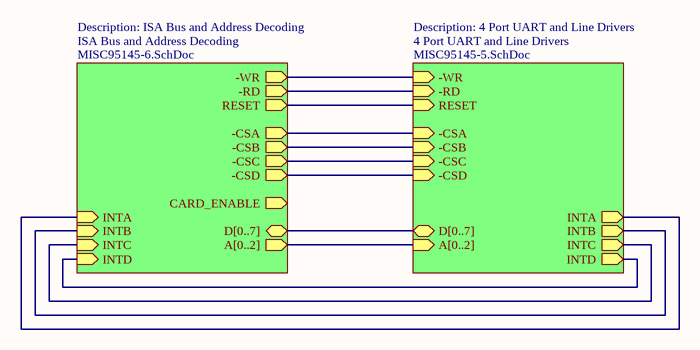
[diagram p0: MISC95145.SchDoc]
# Altium project MISC95145.PRJPCB
3 sheets, 36 parts. Net scope: hierarchical (ports join the sheet entries above them; power ports are global).
Board file: MISC95145.PcbDoc
Sheets:
  MISC95145.SchDoc
    4 Port UART and Line Drivers = MISC95145-5.SchDoc
    ISA Bus and Address Decoding = MISC95145-6.SchDoc

## Sheet MISC95145.SchDoc
size A

### Sub-sheets
4 Port UART and Line Drivers = MISC95145-5.SchDoc: A[0..2] (in), D[0..7] (bidir), -CSA (in), -CSB (in), -CSC (in), -CSD (in), INTA (out), INTB (out), INTC (out), INTD (out), -RD (in), -WR (in), RESET (in)  | Description: 4 Port UART and Line Drivers
ISA Bus and Address Decoding = MISC95145-6.SchDoc: D[0..7] (bidir), -WR (out), -RD (out), RESET (out), A[0..2] (out), -CSA (out), -CSB (out), -CSC (out), -CSD (out), CARD_ENABLE (out), INTB (in), INTC (in), INTD (in), INTA (in)  | Description: ISA Bus and Address Decoding

### Nets
-CSA: sheet 4 Port UART and Line Drivers/-CSA, sheet ISA Bus and Address Decoding/-CSA
-CSB: sheet 4 Port UART and Line Drivers/-CSB, sheet ISA Bus and Address Decoding/-CSB
-CSC: sheet 4 Port UART and Line Drivers/-CSC, sheet ISA Bus and Address Decoding/-CSC
-CSD: sheet 4 Port UART and Line Drivers/-CSD, sheet ISA Bus and Address Decoding/-CSD
-RD: sheet 4 Port UART and Line Drivers/-RD, sheet ISA Bus and Address Decoding/-RD
-WR: sheet 4 Port UART and Line Drivers/-WR, sheet ISA Bus and Address Decoding/-WR
INTA: sheet 4 Port UART and Line Drivers/INTA, sheet ISA Bus and Address Decoding/INTA
INTB: sheet 4 Port UART and Line Drivers/INTB, sheet ISA Bus and Address Decoding/INTB
INTC: sheet 4 Port UART and Line Drivers/INTC, sheet ISA Bus and Address Decoding/INTC
INTD: sheet 4 Port UART and Line Drivers/INTD, sheet ISA Bus and Address Decoding/INTD
RESET: sheet 4 Port UART and Line Drivers/RESET, sheet ISA Bus and Address Decoding/RESET

### Buses and harness runs
bus sheet 4 Port UART and Line Drivers/A[0..2] = sheet ISA Bus and Address Decoding/A[0..2]
bus sheet 4 Port UART and Line Drivers/D[0..7] = sheet ISA Bus and Address Decoding/D[0..7]

### Notes on the sheet
- Title
- Size:
- Date:
- A
- Number:
- Time:
- Revision:
- Sheet
- of
- File:

## Sheet MISC95145-5.SchDoc
size A
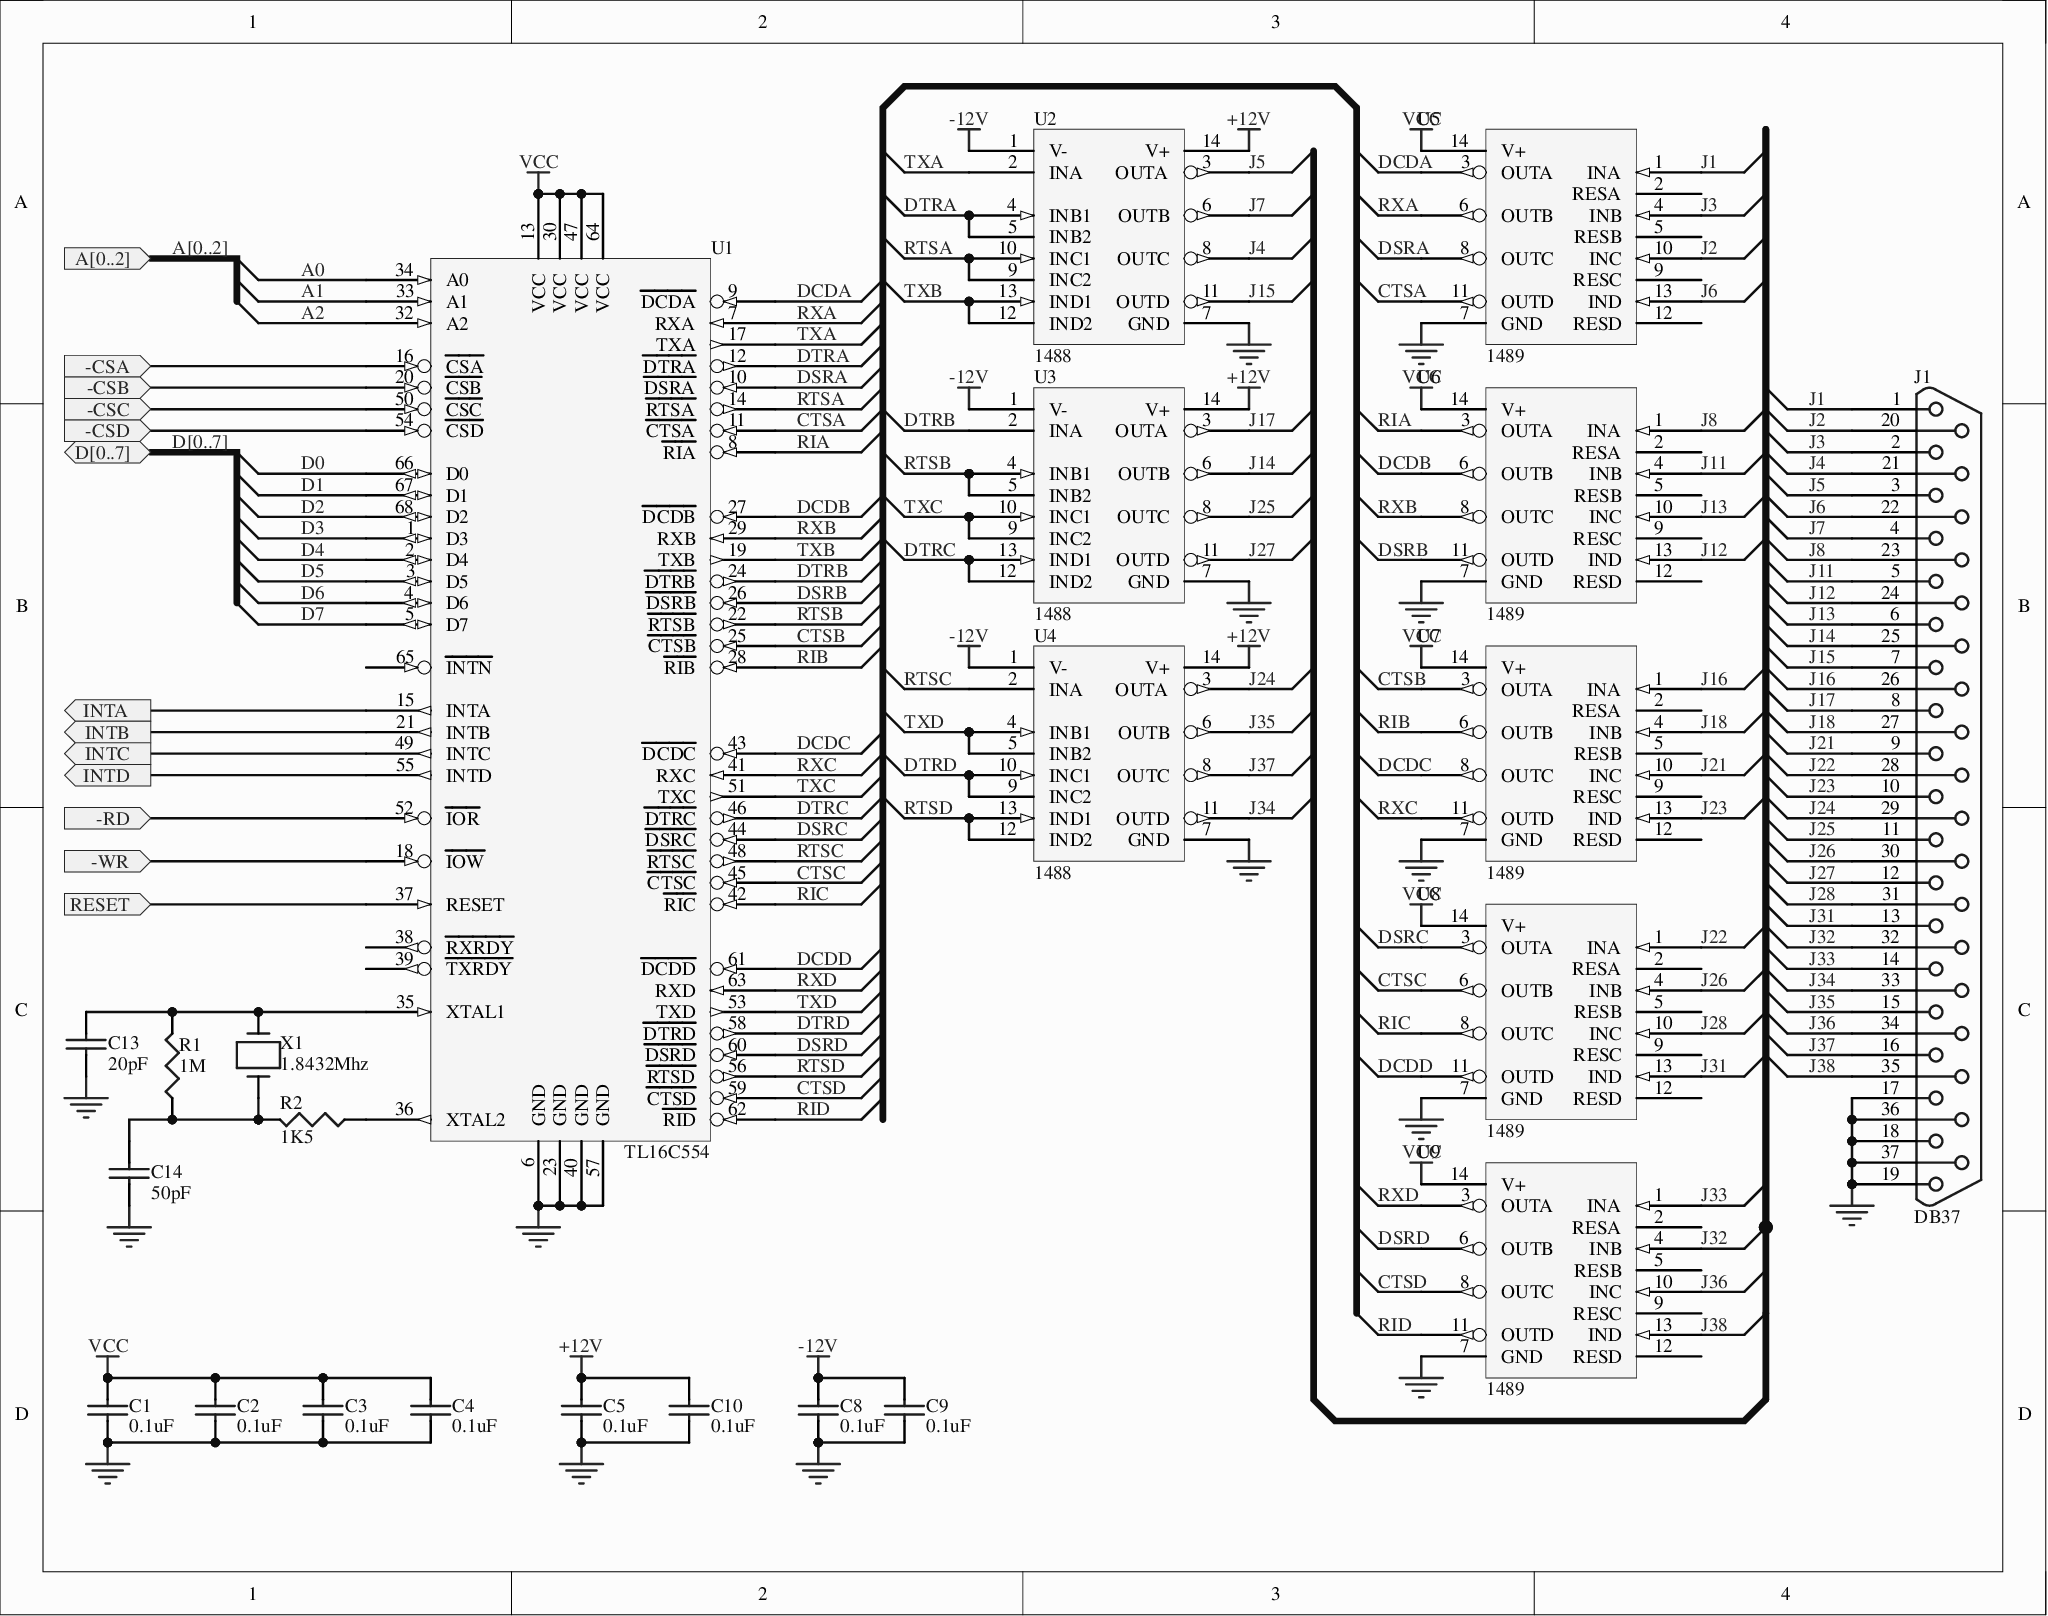
[diagram p1: MISC95145-5.SchDoc]

### Parts
C1  0.1uF  [RAD0.2]
C2  0.1uF  [RAD0.2]
C3  0.1uF  [RAD0.2]
C4  0.1uF  [RAD0.2]
C5  0.1uF  [RAD0.2]
C8  0.1uF  [RAD0.2]
C9  0.1uF  [RAD0.2]
C10  0.1uF  [RAD0.2]
C13  20pF  [RAD0.2]
C14  50pF  [RAD0.2]
J1  DB37  [DB37RA/F]
R1  1M  [AXIAL0.4]
R2  1K5  [AXIAL0.4]
U1  TL16C554  [PGA68X11_SKT]
U2  1488  [DIP14]
U3  1488  [DIP14]
U4  1488  [DIP14]
U5  1489  [DIP14]
U6  1489  [DIP14]
U7  1489  [DIP14]
U8  1489  [DIP14]
U9  1489  [DIP14]
X1  1.8432Mhz  [XTAL1]

### Ports
-CSA (in), -CSB (in), -CSC (in), -CSD (in), -RD (in), -WR (in), A[0..2] (in), D[0..7] (bidir), INTA (out), INTB (out), INTC (out), INTD (out), RESET (in)

### Nets
+12V: C5.1 C10.1 U2.14(V+) U3.14(V+) U4.14(V+)
-12V: C8.1 C9.1 U2.1(V-) U3.1(V-) U4.1(V-)
GND: C1.2 C2.2 C3.2 C4.2 C5.2 C8.2 C9.2 C10.2 C13.2 C14.2 J1.17 J1.18 J1.19 J1.36 J1.37 U1.6(GND) U1.23(GND) U1.40(GND) U1.57(GND) U2.7(GND) U3.7(GND) U4.7(GND) U5.7(GND) U6.7(GND) U7.7(GND) U8.7(GND) U9.7(GND)
VCC: C1.1 C2.1 C3.1 C4.1 U1.13(VCC) U1.30(VCC) U1.47(VCC) U1.64(VCC) U5.14(V+) U6.14(V+) U7.14(V+) U8.14(V+) U9.14(V+)
-CSA: U1.16(~{CSA}) ; port -CSA
-CSB: U1.20(~{CSB}) ; port -CSB
-CSC: U1.50(~{CSC}) ; port -CSC
-CSD: U1.54(~{CSD}) ; port -CSD
-RD: U1.52(~{IOR}) ; port -RD
-WR: U1.18(~{IOW}) ; port -WR
A0: U1.34(A0)
A1: U1.33(A1)
A2: U1.32(A2)
CTSA: U1.11(~{CTSA}) U5.11(OUTD)
CTSB: U1.25(~{CTSB}) U7.3(OUTA)
CTSC: U1.45(~{CTSC}) U8.6(OUTB)
CTSD: U1.59(~{CTSD}) U9.8(OUTC)
D0: U1.66(D0)
D1: U1.67(D1)
D2: U1.68(D2)
D3: U1.1(D3)
D4: U1.2(D4)
D5: U1.3(D5)
D6: U1.4(D6)
D7: U1.5(D7)
DCDA: U1.9(~{DCDA}) U5.3(OUTA)
DCDB: U1.27(~{DCDB}) U6.6(OUTB)
DCDC: U1.43(~{DCDC}) U7.8(OUTC)
DCDD: U1.61(~{DCDD}) U8.11(OUTD)
DSRA: U1.10(~{DSRA}) U5.8(OUTC)
DSRB: U1.26(~{DSRB}) U6.11(OUTD)
DSRC: U1.44(~{DSRC}) U8.3(OUTA)
DSRD: U1.60(~{DSRD}) U9.6(OUTB)
DTRA: U1.12(~{DTRA}) U2.4(INB1) U2.5(INB2)
DTRB: U1.24(~{DTRB}) U3.2(INA)
DTRC: U1.46(~{DTRC}) U3.12(IND2) U3.13(IND1)
DTRD: U1.58(~{DTRD}) U4.9(INC2) U4.10(INC1)
INTA: U1.15(INTA) ; port INTA
INTB: U1.21(INTB) ; port INTB
INTC: U1.49(INTC) ; port INTC
INTD: U1.55(INTD) ; port INTD
J1: J1.1 U5.1(INA)
J2: J1.20 U5.10(INC)
J3: J1.2 U5.4(INB)
J4: J1.21 U2.8(OUTC)
J5: J1.3 U2.3(OUTA)
J6: J1.22 U5.13(IND)
J7: J1.4 U2.6(OUTB)
J8: J1.23 U6.1(INA)
J11: J1.5 U6.4(INB)
J12: J1.24 U6.13(IND)
J13: J1.6 U6.10(INC)
J14: J1.25 U3.6(OUTB)
J15: J1.7 U2.11(OUTD)
J16: J1.26 U7.1(INA)
J17: J1.8 U3.3(OUTA)
J18: J1.27 U7.4(INB)
J21: J1.9 U7.10(INC)
J22: J1.28 U8.1(INA)
J23: J1.10 U7.13(IND)
J24: J1.29 U4.3(OUTA)
J25: J1.11 U3.8(OUTC)
J26: J1.30 U8.4(INB)
J27: J1.12 U3.11(OUTD)
J28: J1.31 U8.10(INC)
J31: J1.13 U8.13(IND)
J32: J1.32 U9.4(INB)
J33: J1.14 U9.1(INA)
J34: J1.33 U4.11(OUTD)
J35: J1.15 U4.6(OUTB)
J36: J1.34 U9.10(INC)
J37: J1.16 U4.8(OUTC)
J38: J1.35 U9.13(IND)
RESET: U1.37(RESET) ; port RESET
RIA: U1.8(~{RIA}) U6.3(OUTA)
RIB: U1.28(~{RIB}) U7.6(OUTB)
RIC: U1.42(~{RIC}) U8.8(OUTC)
RID: U1.62(~{RID}) U9.11(OUTD)
RTSA: U1.14(~{RTSA}) U2.9(INC2) U2.10(INC1)
RTSB: U1.22(~{RTSB}) U3.4(INB1) U3.5(INB2)
RTSC: U1.48(~{RTSC}) U4.2(INA)
RTSD: U1.56(~{RTSD}) U4.12(IND2) U4.13(IND1)
RXA: U1.7(RXA) U5.6(OUTB)
RXB: U1.29(RXB) U6.8(OUTC)
RXC: U1.41(RXC) U7.11(OUTD)
RXD: U1.63(RXD) U9.3(OUTA)
TXA: U1.17(TXA) U2.2(INA)
TXB: U1.19(TXB) U2.12(IND2) U2.13(IND1)
TXC: U1.51(TXC) U3.9(INC2) U3.10(INC1)
TXD: U1.53(TXD) U4.4(INB1) U4.5(INB2)
NetC13_1: C13.1 R1.2 U1.35(XTAL1) X1.2
NetC14_1: C14.1 R1.1 R2.2 X1.1
NetR2_1: R2.1 U1.36(XTAL2)

Not connected (* = marked no-connect by the designer): U1 38(~{RXRDY}) 39(~{TXRDY}) 65(~{INTN})*; U5 2(RESA) 5(RESB) 9(RESC) 12(RESD); U6 2(RESA) 5(RESB) 9(RESC) 12(RESD); U7 2(RESA) 5(RESB) 9(RESC) 12(RESD); U8 2(RESA) 5(RESB) 9(RESC) 12(RESD); U9 2(RESA) 5(RESB) 9(RESC) 12(RESD)

### Buses and harness runs
bus A[0..2] = port A[0..2]
bus D[0..7] = port D[0..7]

### Layout directives
rule Width Constraint [Pref Width = 18mil    Min Width = 18mil    Max Width = 18mil]: GND, VCC

### Notes on the sheet
- Title
- Size:
- Date:
- A
- Number:
- Time:
- Revision:
- Sheet
- of
- File:

### Library data of the parts
C1-C5 C8-C10 = CAP 2M: Capacitor 0.2 pitch; Part Number: C001037; Manufactuer: BC Components; Manufactuer P/N: 2222 370 22104; Capacitance: 0.1µF; Tolerance: 0.05; Voltage-Rated: 100V; Text Field1: CAPACITOR
C13 = CAP 2M: Capacitor 0.2 pitch; Part Number: C001861; Manufactuer: Kemet; Manufactuer P/N: C1206C200J5GACTU; Tolerance: 0.05; Voltage-Rated: 50V; Text Field1: CAPACITOR; Capacitance: 20pF
C14 = CAP 2M: Capacitor 0.2 pitch; Part Number: C001862; Manufactuer: Kemet; Manufactuer P/N: C1206C510J5GACTU; Tolerance: 0.05; Voltage-Rated: 50V; Text Field1: CAPACITOR; Capacitance: 50pF
J1 = DB37: Part Number: J001009; Manufactuer: Norcomp Inc.; Manufactuer P/N: 179-037-412-571
R1 = RES1: Part Number: R002014; Manufactuer: BC; Manufactuer P/N: 2322 245 221.00M; Power: 0.5W; Resistance: 1.00MOhm; Tolerance: 0.1
R2 = RES1: Part Number: R001737; Manufactuer: BC; Manufactuer P/N: 2322 245 221.50K; Power: 0.5W; Resistance: 1.50KOhm; Tolerance: 0.1
U1 = TL16C554: Part Number: U001598; Manufactuer: Maxim; Manufactuer P/N: MX7533JCWE
U2-U4 = 1488_1: TTL-RS232 DRIVER; Part Number: U001659; Manufactuer: Texas Instruments; Manufactuer P/N: MC1488N; Current Rating: 25mA; Voltage-Rated: 9V
U5-U9 = 1489_1: 1489 RS232-TTL CONVERTOR; Part Number: U001701; Manufactuer: Texas Instruments; Manufactuer P/N: MC1489N; Current Rating: 26mA; Voltage-Rated: 5V
X1 = CRYSTAL: Part Number: X001003; Manufactuer: ECS Inc.; Manufactuer P/N: ECS-18-13-1; Load Capacitance: 13pF; Frequency: 1.8432MHz

## Sheet MISC95145-6.SchDoc
size A; Organization: COMPANY_A_____; Address1: xxxxxxxxxxxxxxxxxxxxx; Address2: xxxxxxxxxxxxxx; Address3: NSW; Address4: xxxxxxxxxxxxxx
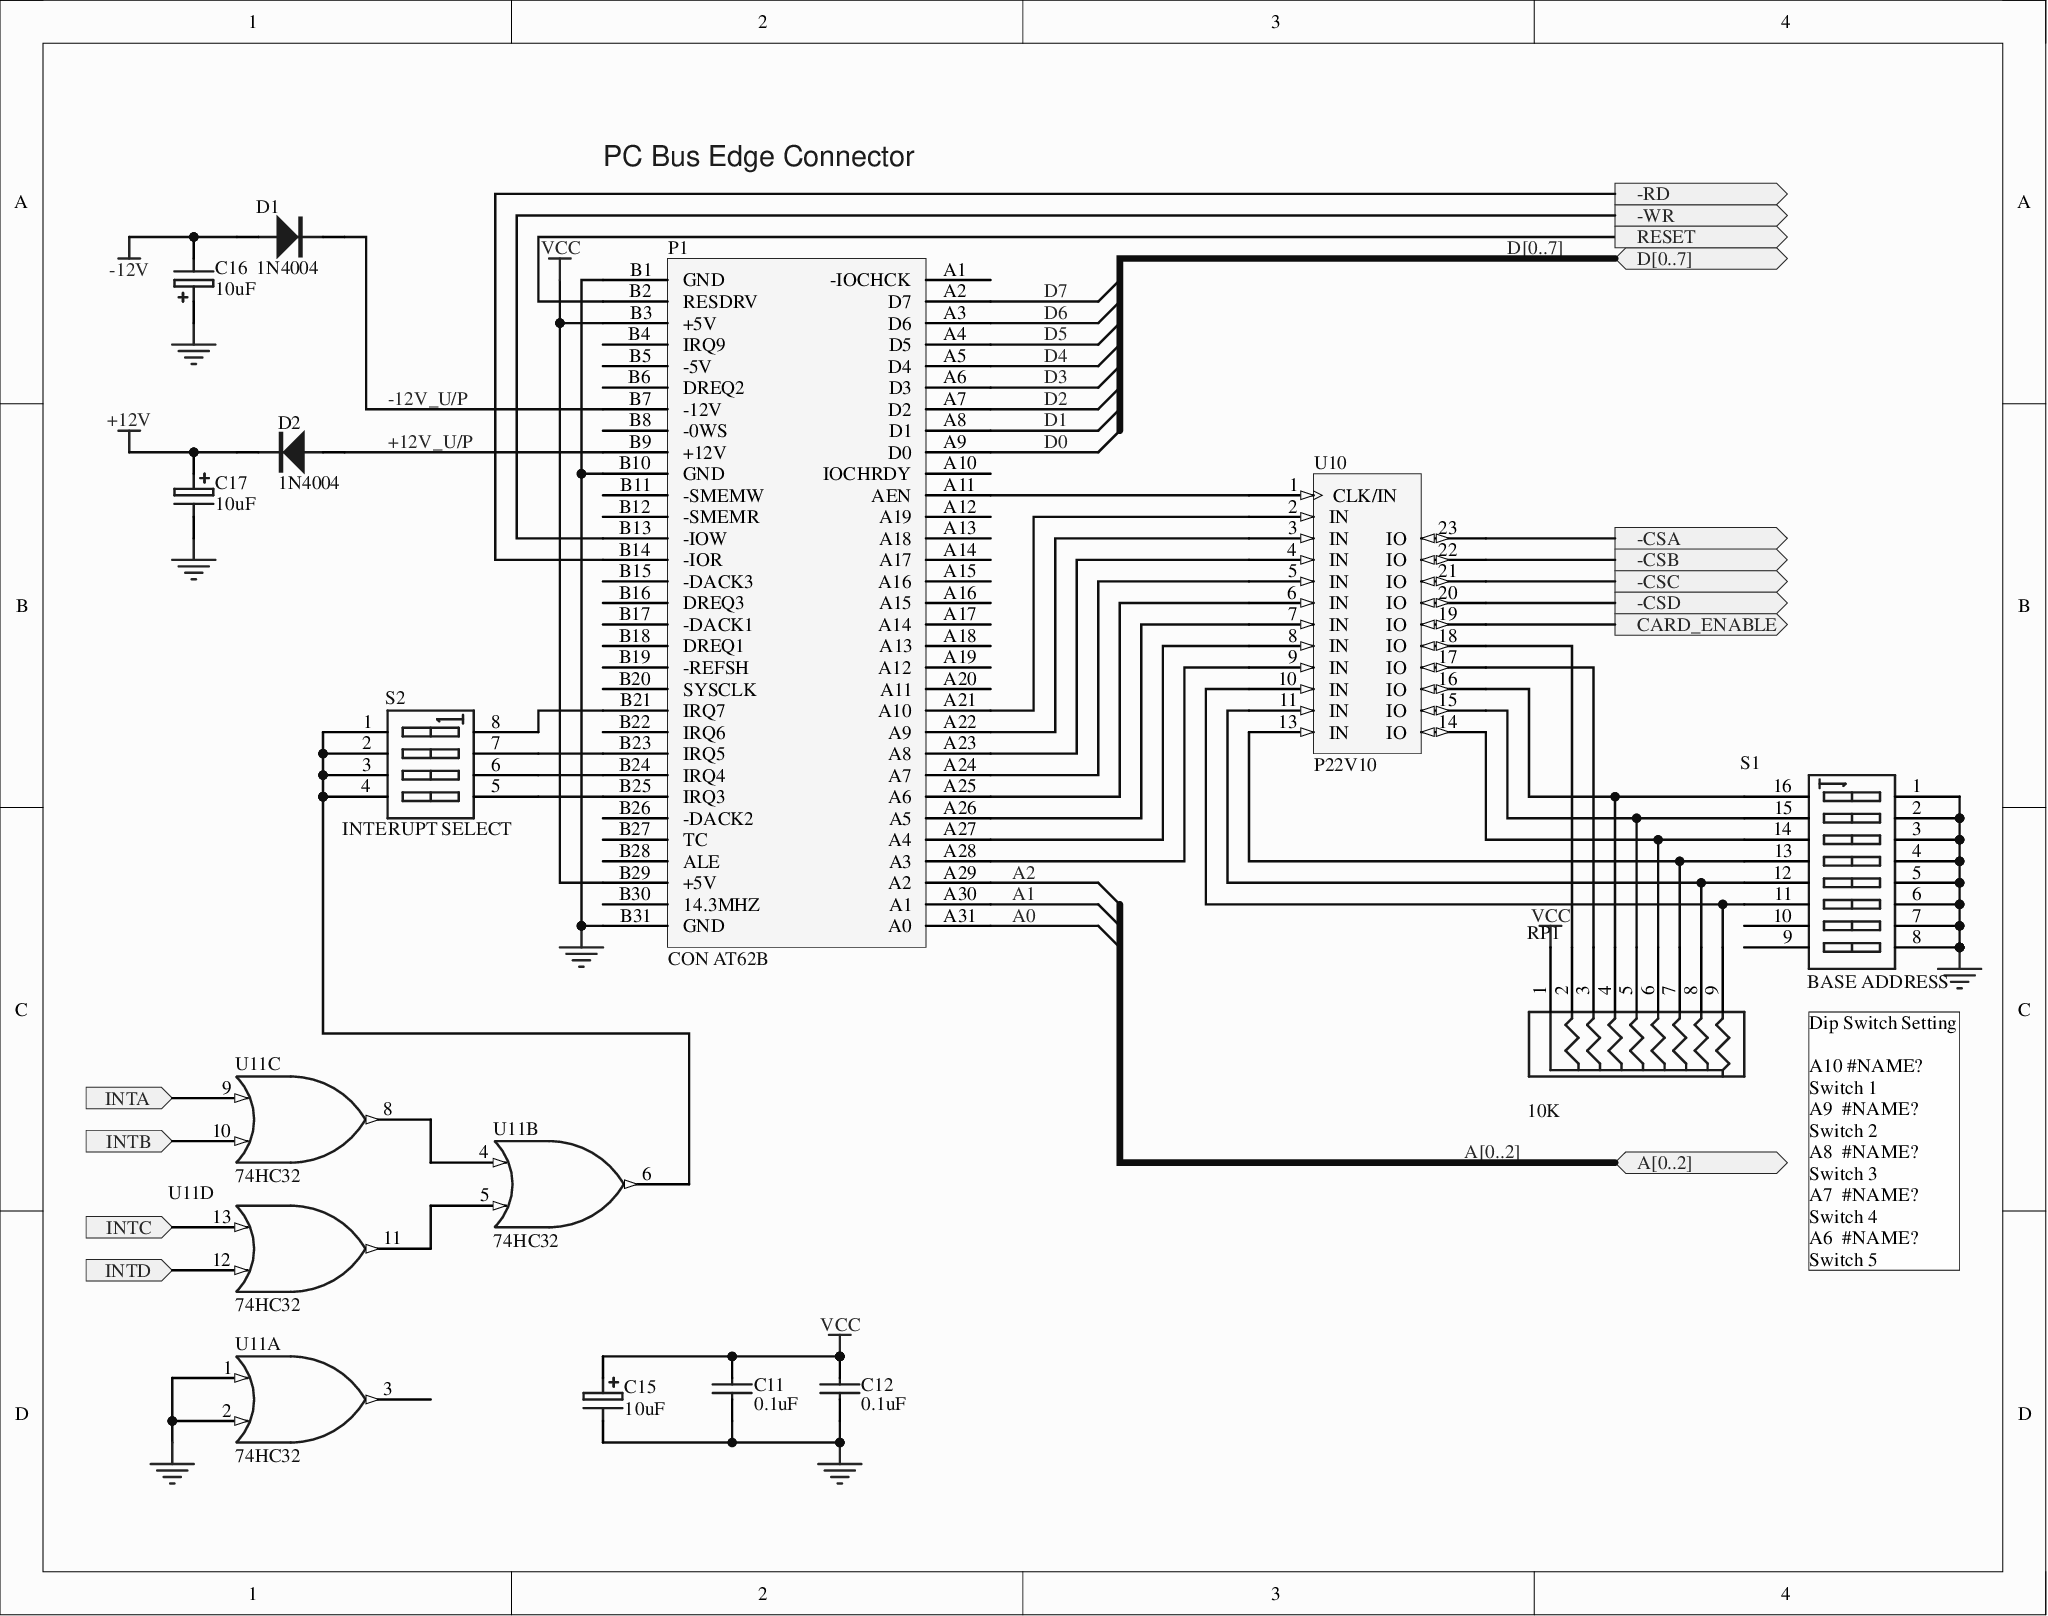
[diagram p2: MISC95145-6.SchDoc]

### Parts
C11  0.1uF  [RAD0.2]
C12  0.1uF  [RAD0.2]
C15  10uF  [TANT 2M/2M]
C16  10uF  [TANT 2M/2M]
C17  10uF  [TANT 2M/2M]
D1  1N4004  [DIODE0.4]
D2  1N4004  [DIODE0.4]
P1  CON AT62B  [ECN-IBMXT]
RP1  10K  [SIP9]
S1  BASE ADDRESS  [DIP16]
S2  INTERUPT SELECT  [DIP8]
U10  P22V10  [SDIP24]
U11  74HC32  [DIP14]  (parts A,B,C,D of 4)

### Ports
-CSA (out), -CSB (out), -CSC (out), -CSD (out), -RD (out), -WR (out), A[0..2] (bidir), CARD_ENABLE (out), D[0..7] (bidir), INTA (in), INTB (in), INTC (in), INTD (in), RESET (out)

### Nets
+12V: C17.1 D2.K
-12V: C16.2 D1.A
GND: C11.2 C12.2 C15.2 C16.1 C17.2 P1.B1(GND) P1.B10(GND) P1.B31(GND) S1.1(A1) S1.2(A2) S1.3(A3) S1.4(A4) S1.5(A5) S1.6(A6) S1.7(A7) S1.8(A8) U10.12(GND) U11.1 U11.2 U11.7(GND)
VCC: C11.1 C12.1 C15.1 P1.B3(+5V) P1.B29(+5V) RP1.1 U10.24(VCC) U11.14(VCC)
+12V_U/P: D2.A P1.B9(+12V)
-12V_U/P: D1.K P1.B7(-12V)
-CSA: U10.23(IO) ; port -CSA
-CSB: U10.22(IO) ; port -CSB
-CSC: U10.21(IO) ; port -CSC
-CSD: U10.20(IO) ; port -CSD
-RD: P1.B14(-IOR) ; port -RD
-WR: P1.B13(-IOW) ; port -WR
A0: P1.A31(A0)
A1: P1.A30(A1)
A2: P1.A29(A2)
CARD_ENABLE: U10.19(IO) ; port CARD_ENABLE
D0: P1.A9(D0)
D1: P1.A8(D1)
D2: P1.A7(D2)
D3: P1.A6(D3)
D4: P1.A5(D4)
D5: P1.A4(D5)
D6: P1.A3(D6)
D7: P1.A2(D7)
INTA: U11.9 ; port INTA
INTB: U11.10 ; port INTB
INTC: U11.13 ; port INTC
INTD: U11.12 ; port INTD
RESET: P1.B2(RESDRV) ; port RESET
NetP1_A11: P1.A11(AEN) U10.1(CLK/IN)
NetP1_A21: P1.A21(A10) U10.2(IN)
NetP1_A22: P1.A22(A9) U10.3(IN)
NetP1_A23: P1.A23(A8) U10.4(IN)
NetP1_A24: P1.A24(A7) U10.5(IN)
NetP1_A25: P1.A25(A6) U10.6(IN)
NetP1_A26: P1.A26(A5) U10.7(IN)
NetP1_A27: P1.A27(A4) U10.8(IN)
NetP1_A28: P1.A28(A3) U10.9(IN)
NetP1_B21: P1.B21(IRQ7) S2.8(B1)
NetP1_B23: P1.B23(IRQ5) S2.7(B2)
NetP1_B24: P1.B24(IRQ4) S2.6(B3)
NetP1_B25: P1.B25(IRQ3) S2.5(B4)
NetRP1_2: RP1.2 U10.18(IO)
NetRP1_3: RP1.3 U10.17(IO)
NetRP1_4: RP1.4 S1.16(B1) U10.16(IO)
NetRP1_5: RP1.5 S1.15(B2) U10.15(IO)
NetRP1_6: RP1.6 S1.14(B3) U10.14(IO)
NetRP1_7: RP1.7 S1.13(B4) U10.13(IN)
NetRP1_8: RP1.8 S1.12(B5) U10.11(IN)
NetRP1_9: RP1.9 S1.11(B6) U10.10(IN)
NetS2_1: S2.1(A1) S2.2(A2) S2.3(A3) S2.4(A4) U11.6
NetU11_4: U11.4 U11.8
NetU11_5: U11.5 U11.11

Not connected (* = marked no-connect by the designer): P1 A1(-IOCHCK) A10(IOCHRDY) A12(A19) A13(A18) A14(A17) A15(A16) A16(A15) A17(A14) A18(A13) A19(A12) A20(A11) B4(IRQ9) B5(-5V) B6(DREQ2) B8(-0WS) B11(-SMEMW) B12(-SMEMR) B15(-DACK3) B16(DREQ3) B17(-DACK1) B18(DREQ1) B19(-REFSH) B20(SYSCLK) B22(IRQ6) B26(-DACK2) B27(TC) B28(ALE) B30(14.3MHZ); S1 9(B8) 10(B7); U11 3

### Buses and harness runs
bus A[0..2] = port A[0..2]
bus D[0..7] = port D[0..7]

### Layout directives
rule Width Constraint [Pref Width = 18mil    Min Width = 18mil    Max Width = 18mil]: +12V, +12V_U/P, -12V, -12V_U/P

### Notes on the sheet
- PC Bus Edge Connector
- Dip Switch Setting
  A10 => Switch 1
  A9  => Switch 2
  A8  => Switch 3
  A7  => Switch 4
  A6  => Switch 5
  A5  => Switch 6
  ---   => Switch 7
  ---   => Switch 8
- Title
- Size:
- Date:
- A
- Number:
- Time:
- Revision:
- Sheet
- of
- File:

### Library data of the parts
C11 C12 = CAP 2M: as C1 on sheet MISC95145-5; Text Field1: CAPACITOR
C15 = ELECTRO RB: Electrolytic Capacitor RB mount; Part Number: C001618; Manufactuer: Panasonic; Manufactuer P/N: ECA-1HHG100; Text Field1: CAPACITOR (ELECTROLYTIC); Capacitance: 10µF; Tolerance: 0.2; Voltage-Rated: 50VDC
C16 C17 = ELECTRO1: Part Number: C001618; Manufactuer: Panasonic; Manufactuer P/N: ECA-1HHG100; Capacitance: 10µF; Tolerance: 0.2; Voltage-Rated: 50VDC
D1 D2 = DIODE: Part Number: X001005; Manufactuer: General Semiconductor; Current Rating: 1A; Voltage Rated: 400V; Manufactuer P/N: 1N4004
P1 = CON AT62B: Part Number: J001027; Manufactuer: EDAC Inc.; Manufactuer P/N: 395-062-520-350
RP1 = RESPACK 8COMMON: RESISTOR NETWORK 8 COMMON RESISTORS; Part Number: R001817; Manufactuer: BC; Manufactuer P/N: 2322 245 2210.0K; Power: 0.5W; Resistance: 10.0KOhm; Tolerance: 0.1
S1 = SW DIP-8: Part Number: S001169; Manufactuer: AMP/Tyco Electronics; Manufactuer P/N: 435640-5; Current Rating: 100mA
S2 = SW DIP-4: Part Number: S001175; Manufactuer: AMP/Tyco Electronics; Manufactuer P/N: 435640-9; Current Rating: 100mA
U10 = P22V10: 24-PIN TTL VERSATILE PAL DEVICE; Part Field 1: CDIP24; Part Number: U001669; Manufactuer: Texas Instruments; Manufactuer P/N: TIBPAL22V10-10CNT; Voltage-Rated: 5V
U11 = SN7432: Quad 2-IN Pos Or G; Part Number: U001680; Manufactuer: Texas Instruments; Manufactuer P/N: SN74HC32N; Voltage-Rated: 5V

## Nets that join several sheets
+12V: MISC95145-5 (5 pins), MISC95145-6 (C17.1 D2.K)
-12V: MISC95145-5 (5 pins), MISC95145-6 (C16.2 D1.A)
GND: MISC95145-5 (27 pins), MISC95145-6 (20 pins)
VCC: MISC95145-5 (13 pins), MISC95145-6 (8 pins)
-CSA: MISC95145-5 (U1.16), MISC95145-6 (U10.23)
-CSB: MISC95145-5 (U1.20), MISC95145-6 (U10.22)
-CSC: MISC95145-5 (U1.50), MISC95145-6 (U10.21)
-CSD: MISC95145-5 (U1.54), MISC95145-6 (U10.20)
-RD: MISC95145-5 (U1.52), MISC95145-6 (P1.B14)
-WR: MISC95145-5 (U1.18), MISC95145-6 (P1.B13)
A0: MISC95145-5 (U1.34), MISC95145-6 (P1.A31)
A1: MISC95145-5 (U1.33), MISC95145-6 (P1.A30)
A2: MISC95145-5 (U1.32), MISC95145-6 (P1.A29)
D0: MISC95145-5 (U1.66), MISC95145-6 (P1.A9)
D1: MISC95145-5 (U1.67), MISC95145-6 (P1.A8)
D2: MISC95145-5 (U1.68), MISC95145-6 (P1.A7)
D3: MISC95145-5 (U1.1), MISC95145-6 (P1.A6)
D4: MISC95145-5 (U1.2), MISC95145-6 (P1.A5)
D5: MISC95145-5 (U1.3), MISC95145-6 (P1.A4)
D6: MISC95145-5 (U1.4), MISC95145-6 (P1.A3)
D7: MISC95145-5 (U1.5), MISC95145-6 (P1.A2)
INTA: MISC95145-5 (U1.15), MISC95145-6 (U11.9)
INTB: MISC95145-5 (U1.21), MISC95145-6 (U11.10)
INTC: MISC95145-5 (U1.49), MISC95145-6 (U11.13)
INTD: MISC95145-5 (U1.55), MISC95145-6 (U11.12)
RESET: MISC95145-5 (U1.37), MISC95145-6 (P1.B2)